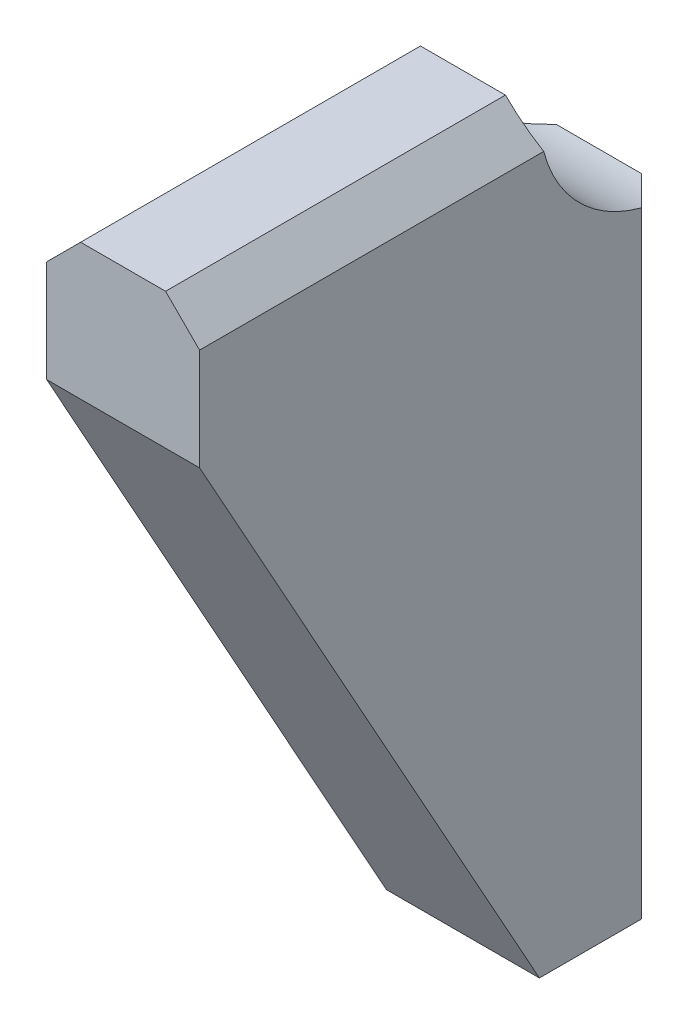
SolidWorks part; units mm, degrees
material "Q235-A"
ref_plane "Front Plane" through (0, 0, 0) normal (0, 0, 1) x (1, 0, 0)
ref_plane "Top Plane" through (0, 0, 0) normal (0, 1, 0) x (1, 0, 0)
ref_plane "Right Plane" through (0, 0, 0) normal (1, 0, 0) x (0, 0, -1)
sketch "Sketch1" plane through (0, 0, 0) normal (1, 0, 0) x (0, 0, -1)
  line L0 (0, 0) -> (0, 180)
  line L1 (-40, 220) -> (-140, 220)
  line L2 (-140, 220) -> (-140, 180)
  line L3 (-140, 180) -> (-40, 0)
  line L4 (-40, 0) -> (0, 0)
  arc A0 (-40, 220) -> (0, 180) centre (0, 220) ccw
  dimension "D1" = 80
  dimension "D2" = 220
  dimension "D3" = 40
  dimension "D4" = 40
  dimension "D5" = 140
extrude "Boss-Extrude1" add sketch "Sketch1" along normal mid plane 45
chamfer "Chamfer1" distance 10 angle 45 4 edges at (-22.5, 90, 0) (22.5, 90, 0) (22.5, 220, 90) (-22.5, 220, 90)
